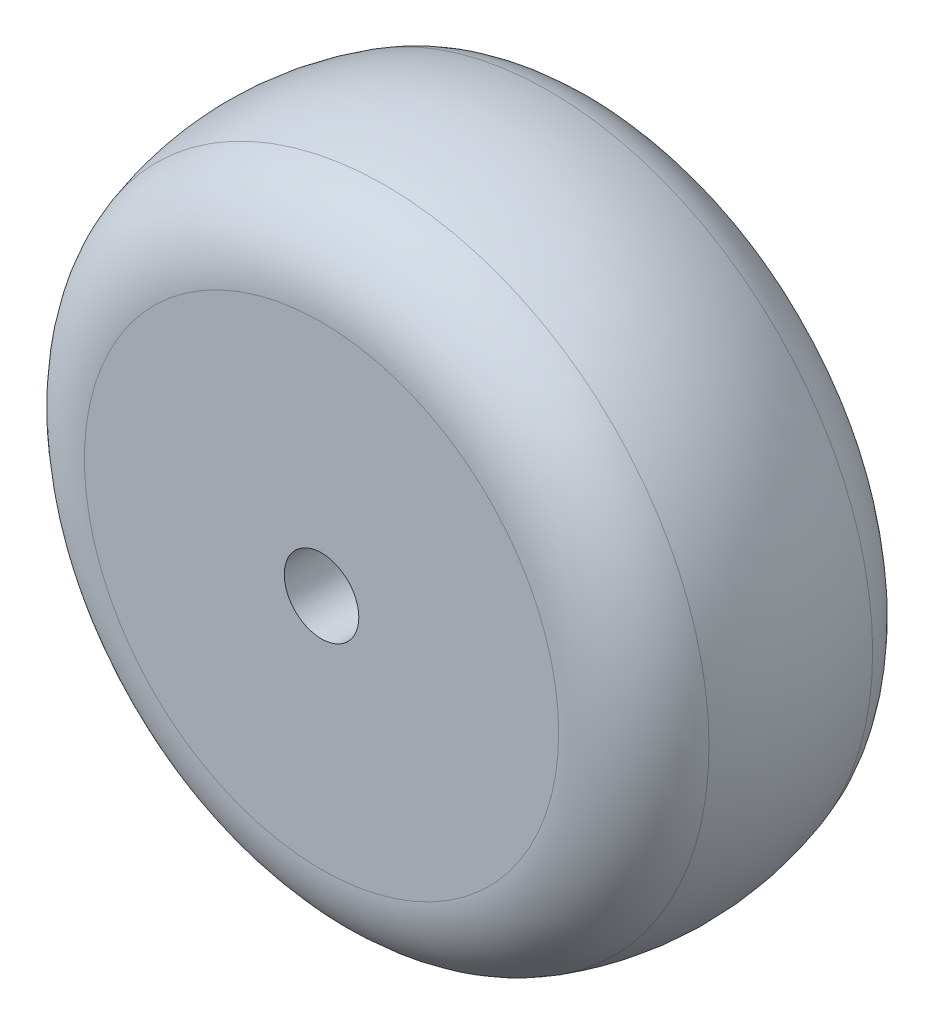
from build123d import *

# Parameters (mm, degrees)
FILLET_1_R = 10


with BuildPart() as part:
    # 草图1 → 旋转1 (revolve)
    with BuildSketch(Plane(origin=(0, 0, 0), x_dir=(1, 0, 0), z_dir=(0, 1, 0))):
        with BuildLine():
            Line((4.1, 16), (32.377155081, 16))
            ThreePointArc((32.377155081, 16), (37, 0), (32.377155081, -16))
            Line((32.377155081, -16), (4.1, -16))
            Line((4.1, -16), (4.1, 16))
        make_face()
    revolve(axis=Axis((0, 0, 0), (0, 0, -1)))

    # 圆角1
    fillet_1_edges = [part.edges().sort_by_distance(p)[0] for p in [
        (-32.377155081, 0, 16),
        (-32.377155081, 0, -16),
    ]]
    fillet(fillet_1_edges, radius=FILLET_1_R)


solid = part.part
